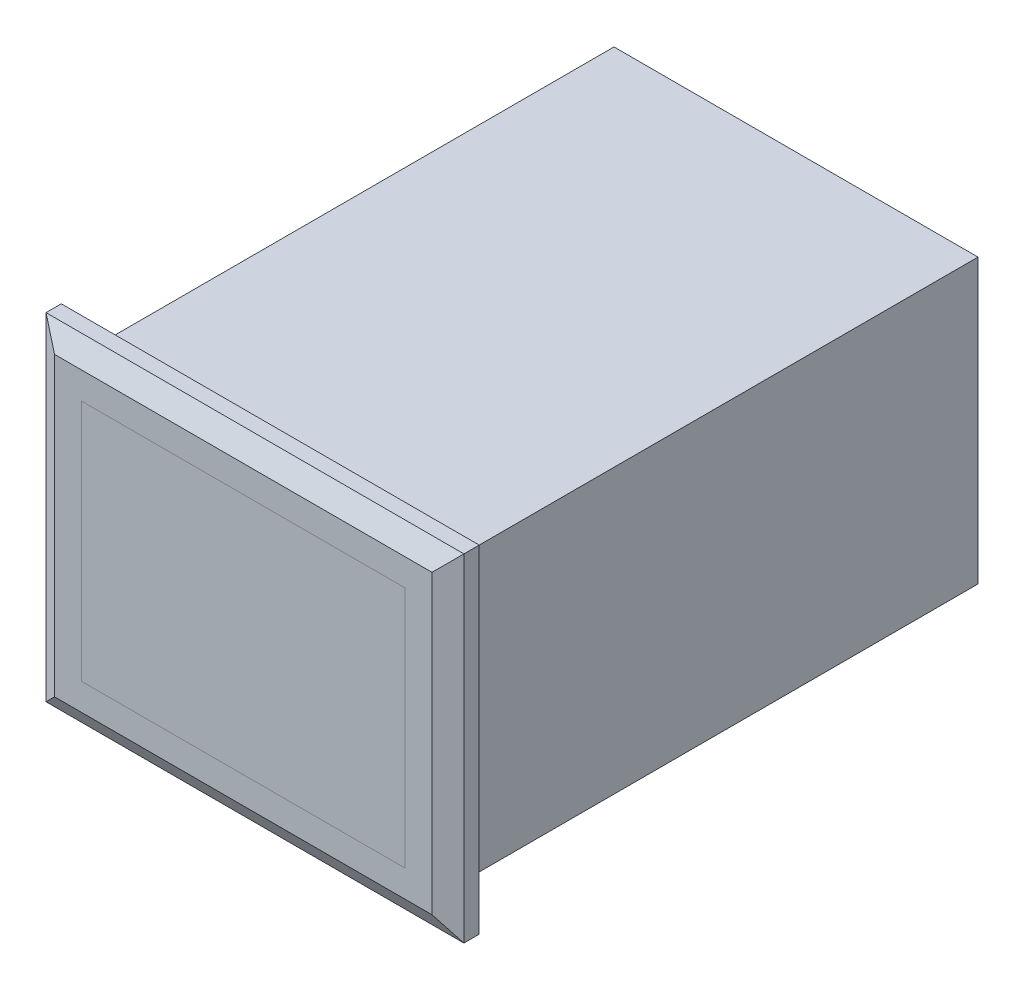
from build123d import *

# Parameters (mm, degrees)
SKETCH1_W           = 27
SKETCH1_H           = 21
BOSS_EXTRUDE1_DEPTH = 39
SKETCH2_W           = 31
SKETCH2_H           = 25
BOSS_EXTRUDE2_DEPTH = 2
CHAMFER1_SIZE       = 1.5
CHAMFER1_SIZE2      = 0.866025404


with BuildPart() as part:
    # Sketch1 → Boss-Extrude1 (new body)
    with BuildSketch(Plane.XY):
        Rectangle(SKETCH1_W, SKETCH1_H)
    extrude(amount=BOSS_EXTRUDE1_DEPTH)

    # Sketch2 → Boss-Extrude2 (add)
    with BuildSketch(Plane.XY.offset(39)):
        Rectangle(SKETCH2_W, SKETCH2_H)
    extrude(amount=BOSS_EXTRUDE2_DEPTH)

    # Chamfer1
    chamfer1_edges = [part.edges().sort_by_distance(p)[0] for p in [
        (15.5, 0, 41),
        (0, 12.5, 41),
        (-15.5, 0, 41),
        (0, -12.5, 41),
    ]]
    chamfer1_side = [part.faces().sort_by_distance(p)[0] for p in [
        (0, 0, 41),
    ]]
    chamfer(chamfer1_edges, length=CHAMFER1_SIZE, length2=CHAMFER1_SIZE2, reference=chamfer1_side[0])


solid = part.part
